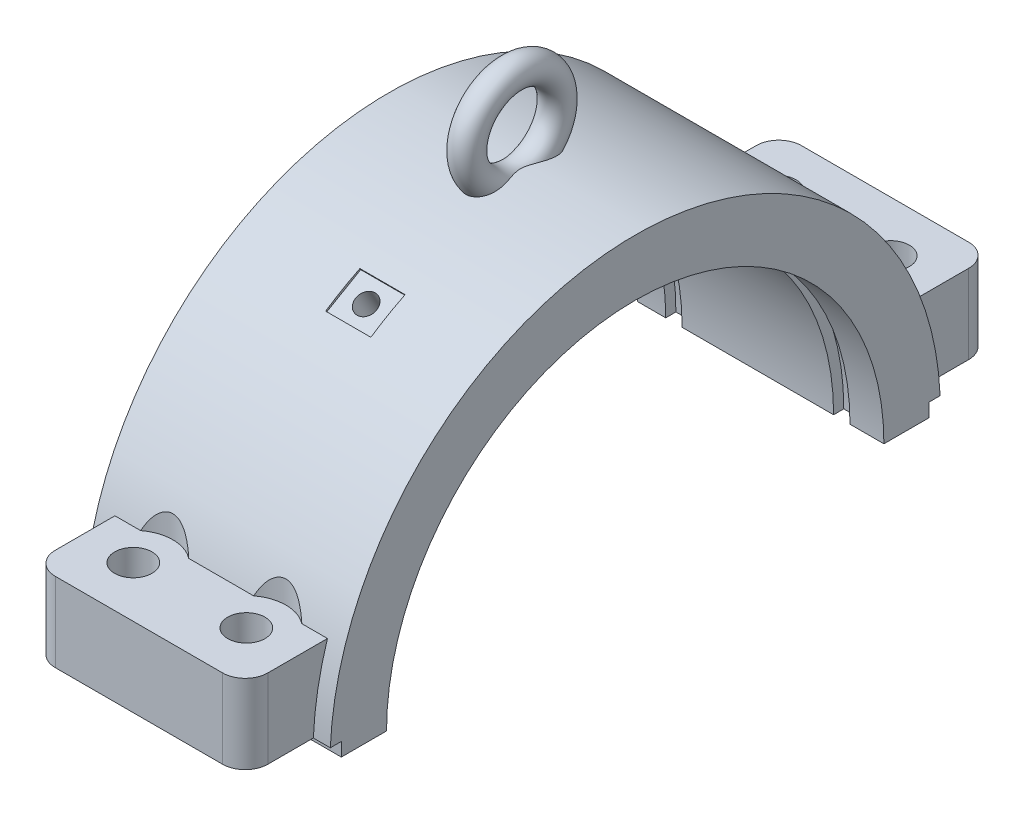
from build123d import *

# Parameters (mm, degrees)
BOSS_EXTRUDE2_DEPTH    = 109
BOSS_EXTRUDE3_DEPTH    = 94
SKETCH5_R              = 16.5
CUT_EXTRUDE1_DEPTH     = 396.126562003
CUT_EXTRUDE2_START     = 82
SKETCH6_R              = 35
CUT_EXTRUDE2_DEPTH     = 19.98039
SKETCH7_W              = 39.278789695
SKETCH7_H              = 17.735547429
CUT_EXTRUDE3_DEPTH     = 441.092035915
FILLET1_R              = 20
FILLET1_OF_MIRROR1_R   = 20
SKETCH8_W              = 14.5
SKETCH8_H              = 9
SKETCH9_R              = 12.5
CUT_EXTRUDE4_START     = 5
CUT_EXTRUDE4_DEPTH     = 20
M20X1_5_TAPPED_HOLE1_D = 18.5


with BuildPart() as part:
    # Sketch1 → Boss-Extrude2 (new, symmetric)
    with BuildSketch(Plane(origin=(0, 0, 0), x_dir=(0, 0, -1), z_dir=(1, 0, 0))):
        with BuildLine():
            Line((-270, 0), (-220, 0))
            ThreePointArc((-220, 0), (0, 220), (220, 0))
            Line((220, 0), (270, 0))
            ThreePointArc((270, 0), (0, 270), (-270, 0))
        make_face()
    extrude(amount=BOSS_EXTRUDE2_DEPTH, both=True)

    # Sketch4 → Boss-Extrude3 (add, symmetric)
    with BuildSketch(Plane(origin=(0, 0, 0), x_dir=(0, 0, -1), z_dir=(1, 0, 0))):
        with BuildLine():
            Line((-330, 12), (-269.733201516, 12))
            ThreePointArc((-269.733201516, 12), (-265.804483526, 47.41283094), (-257.246963053, 82))
            Line((-257.246963053, 82), (-330, 82))
            Line((-330, 82), (-330, 12))
        make_face()
    boss_extrude3 = extrude(amount=BOSS_EXTRUDE3_DEPTH, both=True)

    # Sketch5 → Cut-Extrude1 (cut, symmetric)
    with BuildSketch(Plane(origin=(0, 82, 0), x_dir=(1, 0, 0), z_dir=(0, 1, 0))):
        with Locations(Location((50, -285, 0), (0, 0, 65.380022671))):
            Circle(SKETCH5_R)
        with Locations(Location((-50, -285, 0), (0, 0, 65.380022671))):
            Circle(SKETCH5_R)
    cut_extrude1 = extrude(amount=CUT_EXTRUDE1_DEPTH, both=True, mode=Mode.SUBTRACT)

    # Sketch6 → Cut-Extrude2 (cut)
    with BuildSketch(Plane(origin=(0, 0, 0), x_dir=(1, 0, 0), z_dir=(0, 1, 0)).offset(CUT_EXTRUDE2_START)):
        with Locations((-50, -285)):
            Circle(SKETCH6_R)
        with Locations((50, -285)):
            Circle(SKETCH6_R)
    cut_extrude2 = extrude(amount=CUT_EXTRUDE2_DEPTH, mode=Mode.SUBTRACT)

    # Sketch7 → Cut-Extrude3 (cut, symmetric)
    with BuildSketch(Plane(origin=(0, 0, 0), x_dir=(0, 0, -1), z_dir=(1, 0, 0))):
        with Locations((-279.639394848, 3.132226285)):
            Rectangle(SKETCH7_W, SKETCH7_H)
    cut_extrude3 = extrude(amount=CUT_EXTRUDE3_DEPTH, both=True, mode=Mode.SUBTRACT)

    # Fillet1
    fillet1_edges = [part.edges().sort_by_distance(p)[0] for p in [
        (-94, 47, 330),
        (94, 47, 330),
    ]]
    fillet(fillet1_edges, radius=FILLET1_R)

    # Mirror1: Boss-Extrude3, Cut-Extrude1, Cut-Extrude2, Cut-Extrude3 across plane
    add(boss_extrude3.mirror(Plane.XY))
    add(cut_extrude1.mirror(Plane.XY), mode=Mode.SUBTRACT)
    add(cut_extrude2.mirror(Plane.XY), mode=Mode.SUBTRACT)
    add(cut_extrude3.mirror(Plane.XY), mode=Mode.SUBTRACT)

    # Fillet1 of Mirror1
    fillet1_of_mirror1_edges = [part.edges().sort_by_distance(p)[0] for p in [
        (-94, 47, -330),
        (94, 47, -330),
    ]]
    fillet(fillet1_of_mirror1_edges, radius=FILLET1_OF_MIRROR1_R)

    # Sketch8 → Cut-Revolve1 (revolve, cut)
    with BuildSketch(Plane.XY):
        with Locations((-76.75, 224.5)):
            Rectangle(SKETCH8_W, SKETCH8_H)
        with Locations((71.75, 224.5)):
            Rectangle(SKETCH8_W, SKETCH8_H)
    revolve(axis=Axis((0, 0, 0), (1, 0, 0)), mode=Mode.SUBTRACT)

    # Sketch9 → Revolve1 (revolve)
    with BuildSketch(Plane.XY, mode=Mode.PRIVATE) as revolve1_sk:
        with Locations((0, 340)):
            Circle(SKETCH9_R)
    revolve(revolve1_sk.sketch.rotate(Axis((0, 300, 0), (1, 0, 0)), 340.461761532), axis=Axis((0, 300, 0), (1, 0, 0)))

    # Sketch10 → Cut-Extrude4 (cut, symmetric)
    with BuildSketch(Plane(origin=(0, 0, 0), x_dir=(0, 0, -1), z_dir=(1, 0, 0)).offset(CUT_EXTRUDE4_START)):
        Polygon((-149.155444566, 223.344808214), (-118.844555434, 240.844808214), (-120.844555434, 244.308909829), (-151.155444566, 226.808909829), align=None)
    extrude(amount=CUT_EXTRUDE4_DEPTH, both=True, mode=Mode.SUBTRACT)

    # M20x1.5 Tapped Hole1 (through all)
    with Locations(Plane(origin=(5, 232.094808214, 134), x_dir=(0, -0.5, 0.866025403784), z_dir=(0, 0.866025403784, 0.5))):
        with Locations((0, 0)):
            Hole(M20X1_5_TAPPED_HOLE1_D / 2)


solid = part.part
